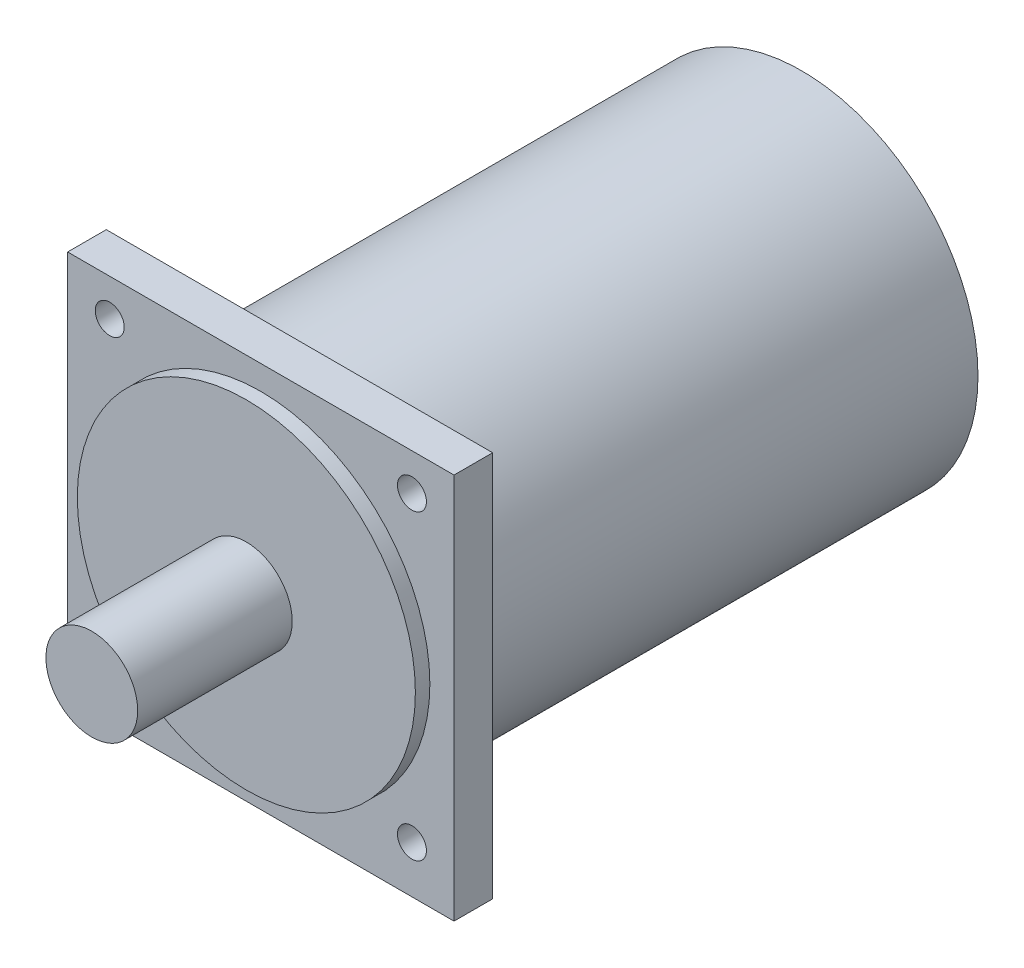
from build123d import *

# Parameters (mm, degrees)
SKETCH_1_W          = 80
SKETCH_1_H          = 80
EXTRUDE_1_DEPTH     = 8
SKETCH_2_R          = 35
EXTRUDE_2_DEPTH     = 3
SKETCH_3_R          = 9.5
EXTRUDE_3_DEPTH     = 32
SKETCH_4_R          = 36.492471365
EXTRUDE_4_DEPTH     = 106
CUT_EXTRUDE_1_REACH = 162.611
SKETCH_5_R          = 3
CHAMFER_1_SIZE      = 2
CHAMFER_1_SIZE2     = 4


with BuildPart() as part:
    # 草图1 → 拉伸1 (new body)
    with BuildSketch(Plane.XY):
        with Locations((40, 40)):
            Rectangle(SKETCH_1_W, SKETCH_1_H)
    extrude(amount=EXTRUDE_1_DEPTH)

    # 草图2 → 拉伸2 (add)
    with BuildSketch(Plane.XY.offset(8)):
        with Locations(Location((40, 40, 0), (0, 0, 180))):
            Circle(SKETCH_2_R)
    extrude(amount=EXTRUDE_2_DEPTH)

    # 草图3 → 拉伸3 (add)
    with BuildSketch(Plane.XY.offset(11)):
        with Locations((40, 40)):
            Circle(SKETCH_3_R)
    extrude(amount=EXTRUDE_3_DEPTH)

    # 草图4 → 拉伸4 (add)
    with BuildSketch(Plane(origin=(0, 0, 0), x_dir=(-1, 0, 0), z_dir=(0, 0, -1))):
        with Locations((-40, 40)):
            Circle(SKETCH_4_R)
    extrude(amount=EXTRUDE_4_DEPTH)

    # 草图5 → 切除-拉伸1 (cut, up to next)
    with BuildSketch(Plane.XY.offset(8), mode=Mode.PRIVATE) as cut_extrude_1_sk1:
        with Locations((8.713677805, 72.344490157)):
            Circle(SKETCH_5_R)
    cut_extrude_1_tool1 = extrude(cut_extrude_1_sk1.sketch, amount=-CUT_EXTRUDE_1_REACH, mode=Mode.PRIVATE) & part.part
    # 草图5 → 切除-拉伸1 (cut, up to next)
    with BuildSketch(Plane.XY.offset(8), mode=Mode.PRIVATE) as cut_extrude_1_sk2:
        with Locations((71.286322195, 72.344490157)):
            Circle(SKETCH_5_R)
    cut_extrude_1_tool2 = extrude(cut_extrude_1_sk2.sketch, amount=-CUT_EXTRUDE_1_REACH, mode=Mode.PRIVATE) & part.part
    # 草图5 → 切除-拉伸1 (cut, up to next)
    with BuildSketch(Plane.XY.offset(8), mode=Mode.PRIVATE) as cut_extrude_1_sk3:
        with Locations((71.286322195, 9.771845767)):
            Circle(SKETCH_5_R)
    cut_extrude_1_tool3 = extrude(cut_extrude_1_sk3.sketch, amount=-CUT_EXTRUDE_1_REACH, mode=Mode.PRIVATE) & part.part
    # 草图5 → 切除-拉伸1 (cut, up to next)
    with BuildSketch(Plane.XY.offset(8), mode=Mode.PRIVATE) as cut_extrude_1_sk4:
        with Locations((8.713677805, 9.771845767)):
            Circle(SKETCH_5_R)
    cut_extrude_1_tool4 = extrude(cut_extrude_1_sk4.sketch, amount=-CUT_EXTRUDE_1_REACH, mode=Mode.PRIVATE) & part.part
    add(cut_extrude_1_tool1.solids().sort_by_distance((8.713678, 72.34449, 8))[0], mode=Mode.SUBTRACT)
    add(cut_extrude_1_tool2.solids().sort_by_distance((71.286322, 72.34449, 8))[0], mode=Mode.SUBTRACT)
    add(cut_extrude_1_tool3.solids().sort_by_distance((71.286322, 9.771846, 8))[0], mode=Mode.SUBTRACT)
    add(cut_extrude_1_tool4.solids().sort_by_distance((8.713678, 9.771846, 8))[0], mode=Mode.SUBTRACT)

    # 倒角1
    chamfer_1_edges = [part.edges().sort_by_distance(p)[0] for p in [
        (76.492471365, 40, -106),
    ]]
    chamfer_1_side = [part.faces().sort_by_distance(p)[0] for p in [
        (76.492471365, 40, -53),
    ]]
    chamfer(chamfer_1_edges, length=CHAMFER_1_SIZE, length2=CHAMFER_1_SIZE2, reference=chamfer_1_side[0])


solid = part.part
